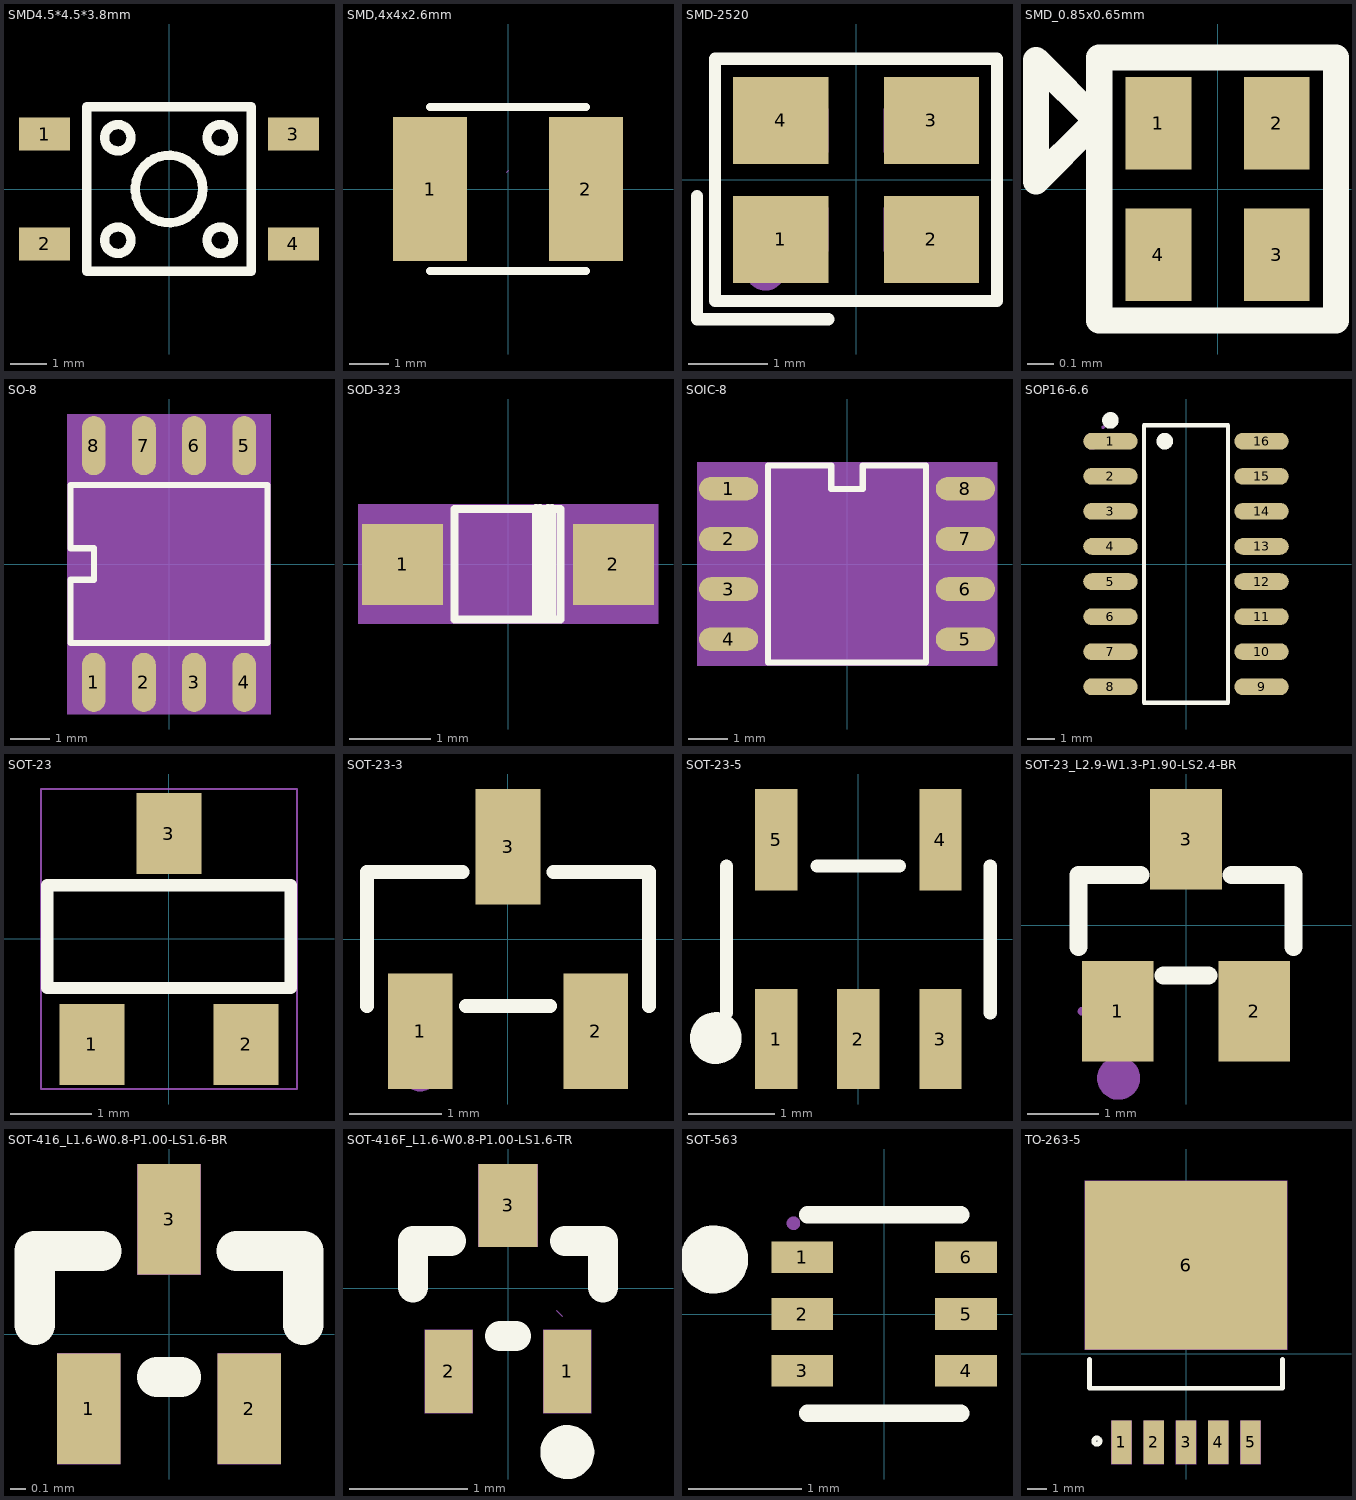
[diagram p0: the footprints below, top view; thin cyan lines are the x and y axes]
# Altium footprint library MISC84456-2.PcbLib: 53 footprints (part 3 of 4)
Each footprint in its own frame and in the unit in brackets; x right, y up, seen from the top. Pads: shape width x height; smd on the part's side, far side on the other; paste and mask are expansions set on the pad; w line width, h text height; cw(c..) or ccw(c..) is an arc to the next point about the centre after c.

## SMD4.5*4.5*3.8mm [mm]
pads (4):
  rect 1.4x0.9 smd: 1(-3.4,1.5) 2(-3.4,-1.5) 3(3.4,1.5) 4(3.4,-1.5)
Top Overlay:
  circle w0.254: c0,0 r0.922
  circle w0.254: c1.4,1.4 r0.361
  circle w0.254: c-1.4,1.4 r0.361
  circle w0.254: c-1.4,-1.4 r0.361
  circle w0.254: c1.4,-1.4 r0.361
  lines w0.254: -2.25,-2.25 2.25,-2.25 2.25,2.25 -2.25,2.25 -2.25,-2.25

## SMD,4x4x2.6mm [mm]
pads (2):
  rect 1.9x3.7 smd: 1(-2,0) 2(2,0)
Top Overlay:
  lines w0.203: -2,-2.1 2,-2.1 ; -2,2.1 2,2.1
Mechanical 15:
  lines w0.003: -0.03,0.43 0.021,0.48

## SMD-2520 [mm]
pads (4):
  rect 1.2x1.1 smd: 1(-0.95,-0.75) 2(0.95,-0.75) 3(0.95,0.75) 4(-0.95,0.75)
Top Overlay:
  lines w0.152: -2.007,-0.201 -2.007,-1.758 -0.351,-1.758 ; -1.779,-1.529 -1.779,1.529 1.779,1.529 1.779,-1.529 -1.779,-1.529
Mechanical 5:
  region: -1.25,0.9 -0.35,0.9 -0.35,0.35 -1.25,0.35
  region: 0.35,0.9 1.25,0.9 1.25,0.35 0.35,0.35
  region: 0.35,-0.35 1.25,-0.35 1.25,-0.9 0.35,-0.9
  region: -1.25,-0.35 -0.35,-0.35 -0.35,-0.9 -1.25,-0.9
Mechanical 6:
  circle w0.06: c-1.25,-1 r0.03
Mechanical 15:
  circle w0.254: c-1.143,-1.143 r0.127

## SMD_0.85x0.65mm [mm]
pads (4):
  rect 0.25x0.35 smd: 1(-0.225,0.25) 2(0.225,0.25) 3(0.225,-0.25) 4(-0.225,-0.25)
Top Overlay:
  lines w0.1: -0.48,0.24 -0.69,0.03 -0.69,0.49 -0.45,0.25 ; -0.48,0.24 -0.48,0.24 ; -0.45,0.25 -0.45,0.25 ; -0.45,-0.5 -0.45,0.5 0.45,0.5 0.45,-0.5 -0.45,-0.5

## SO-8 [mm] "SO-8"
pads (8):
  oval 0.599x1.501 smd: 1(-1.905,-3) 2(-0.635,-3) 3(0.635,-3) 4(1.905,-3) 5(1.905,3) 6(0.635,3) 7(-0.635,3) 8(-1.905,3)
Top Overlay:
  lines w0.152: -2.499,-1.999 -2.499,-0.399 -1.9,-0.399 -1.9,0.399 -2.499,0.399 -2.499,1.999 2.499,1.999 2.499,-1.999 -2.499,-1.999
Mechanical 7:
  text "6" at 0.635,3.254 h1.02
  text "7" at -0.635,3.254 h1.02
  text "4" at 1.905,-2.746 h1.02
  text "8" at -1.905,3.254 h1.02
  text "1" at -1.905,-2.746 h1.02
  text "5" at 1.905,3.254 h1.02
  text "3" at 0.635,-2.746 h1.02
  text "2" at -0.635,-2.746 h1.02
Mechanical 8:
  region: -2.576,-3.8 2.576,-3.8 2.576,3.8 -2.576,3.8
Mechanical 9:
  text "TJA1040T" at 0,1.625 h1.02

## SOD-323 [mm] "SOD-323"
pads (2):
  rect 1.001x1.001 smd: 1(-1.301,-0.005) 2(1.301,-0.005)
Top Overlay:
  lines w0.099: 0.344,-0.683 0.344,0.688 ; 0.394,-0.683 0.394,0.688 ; 0.494,-0.683 0.494,0.688 ; 0.544,-0.683 0.544,0.688 ; -0.658,-0.686 0.645,-0.686 0.645,0.676 -0.658,0.676 -0.658,-0.686
Mechanical 7:
  text "1" at -1.301,0.249 h1.02
  text "2" at 1.301,0.249 h1.02
Mechanical 8:
  region: -1.849,-0.737 1.849,-0.737 1.849,0.737 -1.849,0.737
Mechanical 9:
  text "IN4148" at 1.1,0.045 h1.02
  text ".Designator" at 0.4,0.22 h1.02

## SOIC-8 [mm]
pads (8):
  oval 1.501x0.599 smd: 1(-3,1.905) 2(-3,0.635) 3(-3,-0.635) 4(-3,-1.905) 5(3,-1.905) 6(3,-0.635) 7(3,0.635) 8(3,1.905)
Top Overlay:
  lines w0.152: -1.999,-2.499 -1.999,2.499 -0.399,2.499 -0.399,1.9 0.399,1.9 0.399,2.499 1.999,2.499 1.999,-2.499 -1.999,-2.499
Mechanical 7:
  text "6" at 3.254,-0.635 h1.02
  text "7" at 3.254,0.635 h1.02
  text "4" at -2.746,-1.905 h1.02
  text "8" at 3.254,1.905 h1.02
  text "1" at -2.746,1.905 h1.02
  text "5" at 3.254,-1.905 h1.02
  text "3" at -2.746,-0.635 h1.02
  text "2" at -2.746,0.635 h1.02
Mechanical 8:
  region: -3.8,2.576 -3.8,-2.576 3.8,-2.576 3.8,2.576
Mechanical 9:
  text "TJA1040T" at 1.625,0 h1.02

## SOP16-6.6 [mm]
pads (16):
  oval 1.971x0.602 smd: 1(-2.736,4.445) 2(-2.736,3.175) 3(-2.736,1.905) 4(-2.736,0.635) 5(-2.736,-0.635) 6(-2.736,-1.905) 7(-2.736,-3.175) 8(-2.736,-4.445) 9(2.736,-4.445) 10(2.736,-3.175) 11(2.736,-1.905) 12(2.736,-0.635) 13(2.736,0.635) 14(2.736,1.905) 15(2.736,3.175) 16(2.736,4.445)
Top Overlay:
  circle w0.3: c-0.769,4.445 r0.15
  circle w0.3: c-2.736,5.198 r0.15
  lines w0.152: -1.521,-5.026 1.521,-5.026 1.521,5.026 -1.521,5.026 -1.521,-5.026
Mechanical 5:
  region: -3,4.66 -2.3,4.66 -2.3,4.23 -3,4.23
  pour cut-out: -2.31,4.66 -1.94,4.66 -1.94,4.23 -2.31,4.23
  region: -3,3.39 -2.3,3.39 -2.3,2.96 -3,2.96
  pour cut-out: -2.31,3.39 -1.94,3.39 -1.94,2.96 -2.31,2.96
  region: -3,2.12 -2.3,2.12 -2.3,1.69 -3,1.69
  pour cut-out: -2.31,2.12 -1.94,2.12 -1.94,1.69 -2.31,1.69
  region: -3,0.85 -2.3,0.85 -2.3,0.42 -3,0.42
  pour cut-out: -2.31,0.85 -1.94,0.85 -1.94,0.42 -2.31,0.42
  region: -3,-0.42 -2.3,-0.42 -2.3,-0.85 -3,-0.85
  pour cut-out: -2.31,-0.42 -1.94,-0.42 -1.94,-0.85 -2.31,-0.85
  region: -3,-1.69 -2.3,-1.69 -2.3,-2.12 -3,-2.12
  pour cut-out: -2.31,-1.69 -1.94,-1.69 -1.94,-2.12 -2.31,-2.12
  region: -3,-2.96 -2.3,-2.96 -2.3,-3.39 -3,-3.39
  pour cut-out: -2.31,-2.96 -1.94,-2.96 -1.94,-3.39 -2.31,-3.39
  region: -3,-4.23 -2.3,-4.23 -2.3,-4.66 -3,-4.66
  pour cut-out: -2.31,-4.23 -1.94,-4.23 -1.94,-4.66 -2.31,-4.66
  region: 3,4.66 2.3,4.66 2.3,4.23 3,4.23
  pour cut-out: 2.31,4.66 1.94,4.66 1.94,4.23 2.31,4.23
  region: 3,3.39 2.3,3.39 2.3,2.96 3,2.96
  pour cut-out: 2.31,3.39 1.94,3.39 1.94,2.96 2.31,2.96
  region: 3,2.12 2.3,2.12 2.3,1.69 3,1.69
  pour cut-out: 2.31,2.12 1.94,2.12 1.94,1.69 2.31,1.69
  region: 3,0.85 2.3,0.85 2.3,0.42 3,0.42
  pour cut-out: 2.31,0.85 1.94,0.85 1.94,0.42 2.31,0.42
  region: 3,-0.42 2.3,-0.42 2.3,-0.85 3,-0.85
  pour cut-out: 2.31,-0.42 1.94,-0.42 1.94,-0.85 2.31,-0.85
  region: 3,-1.69 2.3,-1.69 2.3,-2.12 3,-2.12
  pour cut-out: 2.31,-1.69 1.94,-1.69 1.94,-2.12 2.31,-2.12
  region: 3,-2.96 2.3,-2.96 2.3,-3.39 3,-3.39
  pour cut-out: 2.31,-2.96 1.94,-2.96 1.94,-3.39 2.31,-3.39
  region: 3,-4.23 2.3,-4.23 2.3,-4.66 3,-4.66
  pour cut-out: 2.31,-4.23 1.94,-4.23 1.94,-4.66 2.31,-4.66
Mechanical 6:
  circle w0.06: c-3,4.95 r0.03
Mechanical 15:
  circle w0.3: c-3.4,4.445 r0.15

## SOT-23 [mm] "SOT-23"
pads (3):
  rect 0.8x1 smd: 1(-0.95,-1.3) 2(0.95,-1.3) 3(0,1.3)
Top Overlay:
  lines w0.152: -1.5,-0.605 1.5,-0.605 1.5,0.665 -1.5,0.665 -1.5,-0.605
Mechanical 7:
  text "1" at -1.204,-1.3 h1.02
  text "3" at -0.254,1.3 h1.02
  text "2" at 0.696,-1.3 h1.02
Mechanical 8:
  lines w0.025: -1.576,-1.85 1.576,-1.85 1.576,1.85 -1.576,1.85 -1.576,-1.85
Mechanical 9:
  text "MMBT3904" at -1.35,-0.025 h1.02
  text ".Designator" at -0.075,0.45 h1.02

## SOT-23-3 [mm]
pads (3):
  rect 0.7x1.25 smd: 1(-0.95,-1) 2(0.95,-1) 3(0,1)
Top Overlay:
  lines w0.152: -1.526,-0.726 -1.526,0.726 -0.495,0.726 ; -0.455,-0.726 0.455,-0.726 ; 0.495,0.726 1.526,0.726 1.526,-0.726
Mechanical 5:
  pour cut-out: -0.215,0.86 0.215,0.86 0.215,0.64 -0.215,0.64
  region: -0.215,0.85 0.215,0.85 0.215,1.15 -0.215,1.15
  pour cut-out: 0.735,-0.64 1.165,-0.64 1.165,-0.86 0.735,-0.86
  region: 0.735,-0.85 1.165,-0.85 1.165,-1.15 0.735,-1.15
  pour cut-out: -1.165,-0.64 -0.735,-0.64 -0.735,-0.86 -1.165,-0.86
  region: -1.165,-0.85 -0.735,-0.85 -0.735,-1.15 -1.165,-1.15
Mechanical 15:
  circle w0.2: c-0.95,-1.45 r0.1

## SOT-23-5 [mm]
pads (5):
  rect 0.49x1.157 smd: 1(-0.95,-1.154) 2(0,-1.154) 3(0.95,-1.154)
  rect 0.49x1.175 smd: 4(0.95,1.154) 5(-0.95,1.154)
Top Overlay:
  circle w0.3: c-1.651,-1.143 r0.15
  lines w0.152: -1.526,-0.851 -1.526,0.851 ; -0.476,0.851 0.476,0.851 ; 1.526,-0.851 1.526,0.851
Mechanical 5:
  pour cut-out: -1.125,0.74 -1.125,1.01 -0.775,1.01 -0.775,0.74
  region: -1.125,1 -1.125,1.4 -0.775,1.4 -0.775,1
  pour cut-out: 0.775,0.74 0.775,1.01 1.125,1.01 1.125,0.74
  region: 0.775,1 0.775,1.4 1.125,1.4 1.125,1
  pour cut-out: 0.775,-1.01 0.775,-0.74 1.125,-0.74 1.125,-1.01
  region: 0.775,-1.4 0.775,-1 1.125,-1 1.125,-1.4
  pour cut-out: -0.175,-1.01 -0.175,-0.74 0.175,-0.74 0.175,-1.01
  region: -0.175,-1.4 -0.175,-1 0.175,-1 0.175,-1.4

## SOT-23_L2.9-W1.3-P1.90-LS2.4-BR [mm]
pads (3):
  rect 1x1.4 smd: 1(-0.95,-1.2) 2(0.95,-1.2) 3(0,1.2)
Top Overlay:
  lines w0.254: -1.5,-0.3 -1.5,0.7 -0.636,0.7 ; -0.314,-0.7 0.314,-0.7 ; 0.636,0.7 1.5,0.7 1.5,-0.3
Mechanical 5:
  region: -1.192,-1 -0.707,-1 -0.707,-1.2 -1.192,-1.2
  pour cut-out: -1.192,-0.64 -0.707,-0.64 -0.707,-1.01 -1.192,-1.01
  region: 0.708,-1 1.193,-1 1.193,-1.2 0.708,-1.2
  pour cut-out: 0.708,-0.64 1.193,-0.64 1.193,-1.01 0.708,-1.01
  region: -0.242,1.2 0.243,1.2 0.243,1 -0.242,1
  pour cut-out: -0.242,1.01 0.243,1.01 0.243,0.64 -0.242,0.64
Mechanical 6:
  circle w0.06: c-1.45,-1.2 r0.03
Mechanical 15:
  circle w0.3: c-0.94,-2.134 r0.15

## SOT-416_L1.6-W0.8-P1.00-LS1.6-BR [mm]
pads (3):
  rect 0.4x0.7 smd: 1(-0.508,-0.473) 2(0.508,-0.473) 3(0,0.727)
Top Overlay:
  lines w0.254: -0.85,0.059 -0.85,0.527 -0.428,0.527 ; -0.077,-0.273 0.077,-0.273 ; 0.428,0.527 0.85,0.527 0.85,0.059
Mechanical 5:
  region: -0.308,-0.123 -0.308,-0.823 -0.708,-0.823 -0.708,-0.123
  region: 0.708,-0.123 0.708,-0.823 0.308,-0.823 0.308,-0.123
  region: 0.2,1.077 0.2,0.377 -0.2,0.377 -0.2,1.077

## SOT-416F_L1.6-W0.8-P1.00-LS1.6-TR [mm]
pads (3):
  rect 0.4x0.7 smd: 1(0.5,-0.7) 2(-0.5,-0.7)
  rect 0.5x0.7 smd: 3(0,0.7)
Top Overlay:
  circle w0.254: c0.5,-1.38 r0.101
  lines w0.254: -0.8,0.009 -0.8,0.4 -0.481,0.4 ; -0.068,-0.4 0.068,-0.4 ; 0.481,0.4 0.8,0.4 0.8,0.009
Mechanical 5:
  region: 0.25,1.05 0.25,0.35 -0.25,0.35 -0.25,1.05
  region: 0.701,-0.349 0.701,-1.05 0.299,-1.05 0.299,-0.349
  region: -0.299,-0.349 -0.299,-1.05 -0.701,-1.05 -0.701,-0.349
Mechanical 15:
  lines w0.003: 0.408,-0.184 0.459,-0.235

## SOT-563 [mm]
pads (6):
  rect 0.545x0.28 smd: 1(-0.723,0.5) 2(-0.723,0) 3(-0.723,-0.5) 4(0.723,-0.5) 5(0.723,0) 6(0.723,0.5)
Top Overlay:
  circle w0.3: c-1.5,0.481 r0.15
  lines w0.152: -0.676,-0.876 0.676,-0.876 ; -0.676,0.876 0.676,0.876
Mechanical 5:
  region: 0.811,0.612 0.811,0.387 0.586,0.387 0.586,0.612
  region: 0.811,0.112 0.811,-0.112 0.586,-0.112 0.586,0.112
  region: 0.811,-0.388 0.811,-0.613 0.586,-0.613 0.586,-0.388
  region: -0.586,-0.388 -0.586,-0.613 -0.811,-0.613 -0.811,-0.388
  region: -0.586,0.112 -0.586,-0.112 -0.811,-0.112 -0.811,0.112
  region: -0.586,0.612 -0.586,0.387 -0.811,0.387 -0.811,0.612
Mechanical 6:
  circle w0.06: c-0.8,0.8 r0.03

## TO-263-5 [mil]
pads (6):
  rect 42.1x90 smd: 1(-134,-183.77) 2(-67,-183.77) 3(0,-183.77) 4(67,-183.77) 5(134,-183.77)
  rect 419.68x350 smd: 6(0,183.77)
Top Overlay:
  circle w10: c-185,-181.27 r6.5
  lines w10: -200,-11.27 -200,-71.77 200,-71.77 200,-11.27
Mechanical 5:
  region: -209.84,8.77 -209.84,358.77 209.84,358.77 209.84,8.77
  region: 112.95,-228.77 112.95,-138.77 155.05,-138.77 155.05,-228.77
  region: 45.95,-228.77 45.95,-138.77 88.05,-138.77 88.05,-228.77
  region: -88.05,-228.77 -88.05,-138.77 -45.95,-138.77 -45.95,-228.77
  region: -21.05,-228.77 -21.05,-138.77 21.05,-138.77 21.05,-228.77
  region: -155.05,-228.77 -155.05,-138.77 -112.95,-138.77 -112.95,-228.77
Mechanical 15:
  lines w0.1: -19.75,65.77 -17.75,63.77